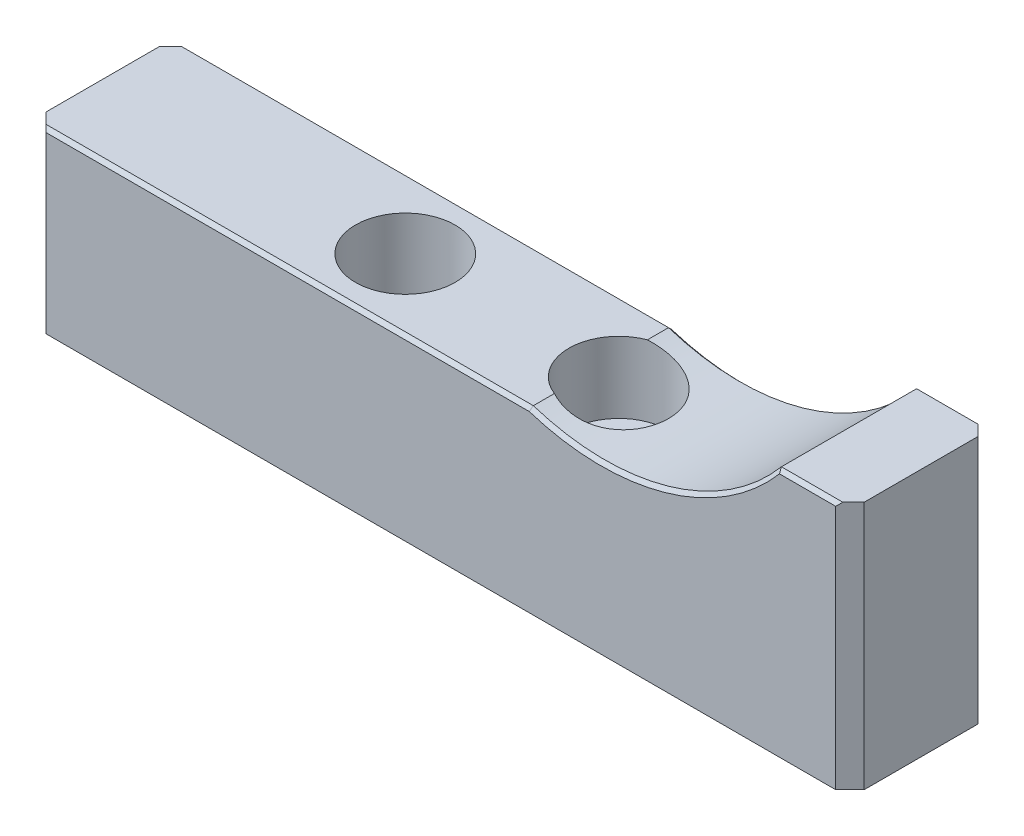
from build123d import *

# Parameters (mm, degrees)
EXTRUDE_1_DEPTH     = 20
SKETCH_4_R          = 7
CUT_EXTRUDE_1_DEPTH = 20
SKETCH_5_R          = 4.5
CUT_EXTRUDE_2_DEPTH = 20
CHAMFER_1_SIZE      = 2
CHAMFER_2_SIZE      = 0.5


with BuildPart() as part:
    # 草图2 → 凸台-拉伸1 (new body)
    with BuildSketch(Plane.XY):
        with BuildLine():
            Line((0, 0), (0, 25))
            Line((0, 25), (70, 25))
            ThreePointArc((70, 25), (88.959441577, 24.682639084), (104.868973518, 35))
            Line((104.868973518, 35), (115, 35))
            Line((115, 35), (115, 0))
            Line((115, 0), (0, 0))
        make_face()
    extrude(amount=EXTRUDE_1_DEPTH)

    # 草图4 → 切除-拉伸1 (cut)
    with BuildSketch(Plane(origin=(0, 35, 0), x_dir=(1, 0, 0), z_dir=(0, 1, 0))):
        with Locations(Location((42.5, -10, 0), (0, 0, 180))):
            Circle(SKETCH_4_R)
        with Locations(Location((72.5, -10, 0), (0, 0, 180))):
            Circle(SKETCH_4_R)
    extrude(amount=-CUT_EXTRUDE_1_DEPTH, mode=Mode.SUBTRACT)

    # 草图5 → 切除-拉伸2 (cut)
    with BuildSketch(Plane(origin=(0, 15, 0), x_dir=(1, 0, 0), z_dir=(0, 1, 0))):
        with Locations(Location((42.5, -10, 0), (0, 0, 180))):
            Circle(SKETCH_5_R)
        with Locations(Location((72.5, -10, 0), (0, 0, 180))):
            Circle(SKETCH_5_R)
    extrude(amount=-CUT_EXTRUDE_2_DEPTH, mode=Mode.SUBTRACT)

    # 倒角1
    chamfer_1_edges = [part.edges().sort_by_distance(p)[0] for p in [
        (0, 12.5, 20),
        (0, 12.5, 0),
        (115, 17.5, 20),
        (115, 17.5, 0),
    ]]
    chamfer(chamfer_1_edges, length=CHAMFER_1_SIZE)

    # 倒角2
    chamfer_2_edges = [part.edges().sort_by_distance(p)[0] for p in [
        (88.959441577, 24.682639084, 20),
        (36, 25, 20),
        (108.934486759, 35, 20),
        (108.934486759, 35, 0),
        (36, 25, 0),
        (88.959441577, 24.682639084, 0),
    ]]
    chamfer(chamfer_2_edges, length=CHAMFER_2_SIZE)


solid = part.part
